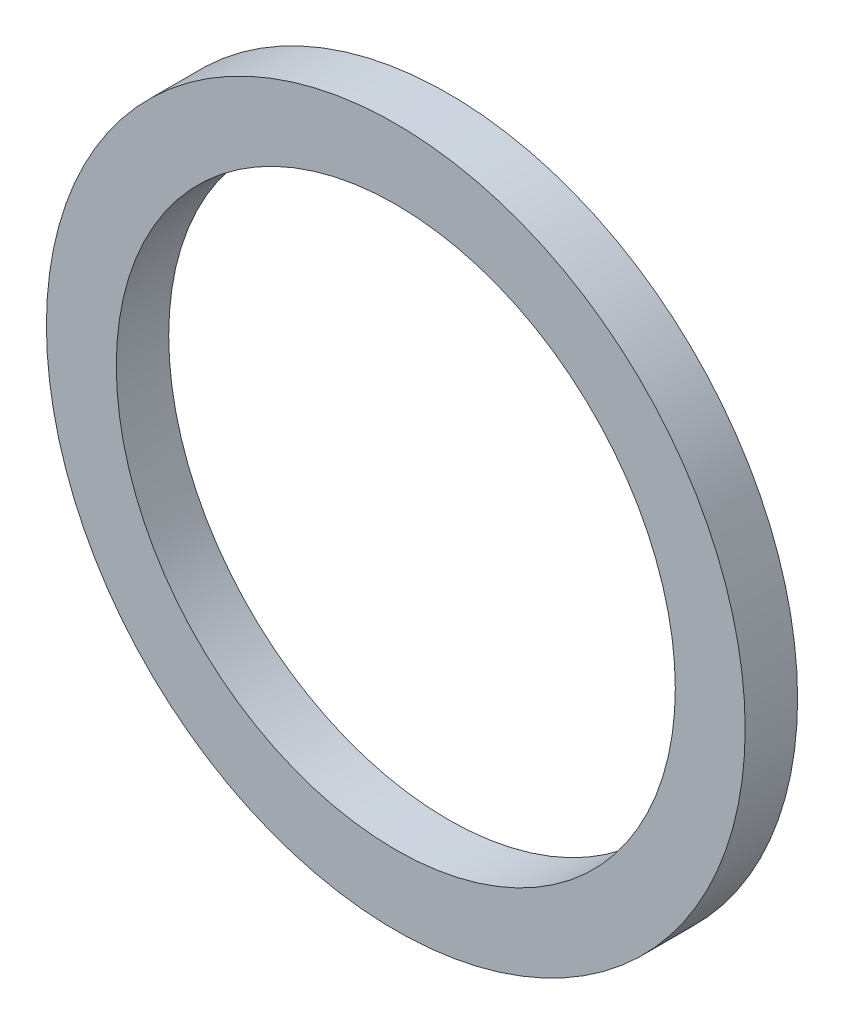
from build123d import *

# Parameters (mm, degrees)
SKETCH_1_R      = 10
SKETCH_1_R_2    = 8
EXTRUDE_1_DEPTH = 1.5


with BuildPart() as part:
    # 草图1 → 凸台-拉伸1 (new body)
    with BuildSketch(Plane.XY):
        Circle(SKETCH_1_R)
        Circle(SKETCH_1_R_2, mode=Mode.SUBTRACT)
    extrude(amount=EXTRUDE_1_DEPTH)


solid = part.part
